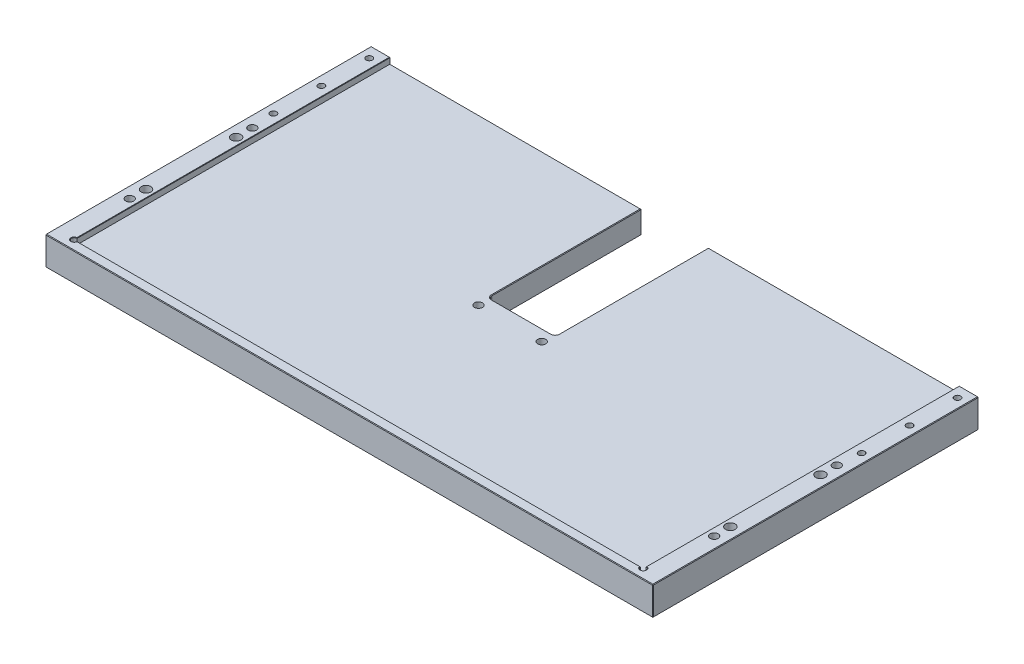
SolidWorks part; units mm, degrees
material "Al6061"
ref_plane "Front" through (0, 0, 0) normal (0, 0, 1) x (1, 0, 0)
ref_plane "Top" through (0, 0, 0) normal (0, 1, 0) x (1, 0, 0)
ref_plane "Right" through (0, 0, 0) normal (1, 0, 0) x (0, 0, -1)
sketch "草图1" plane through (0, 0, 0) normal (0, 1, 0) x (1, 0, 0)
  line L1 (-158.5, 85) -> (158.5, 85)
  line L2 (-158.5, 85) -> (-158.5, -85)
  line L3 (-158.5, -85) -> (158.5, -85)
  line L4 (158.5, 85) -> (158.5, -85)
  line L5 (-158.5, 85) -> (158.5, -85) construction
  line L6 (-158.5, -85) -> (158.5, 85) construction
  point P0 (0, 0)
  dimension "D1" = 317
  dimension "D2" = 170
extrude "凸台-拉伸1" add sketch "草图1" along normal blind 15
sketch "草图2" plane through (0, 15, 0) normal (0, 1, 0) x (1, 0, 0)
  line L0 (158.5, 85) -> (-158.5, 85) construction
  line L1 (-148.5, 250) -> (148.5, 250)
  line L2 (-148.5, 250) -> (-148.5, -80)
  line L3 (-148.5, -80) -> (148.5, -80)
  line L4 (148.5, 250) -> (148.5, -80)
  line L5 (-148.5, 250) -> (148.5, -80) construction
  line L6 (-148.5, -80) -> (148.5, 250) construction
  line L7 (158.5, -85) -> (158.5, 85) construction
  line L8 (-158.5, -85) -> (158.5, -85) construction
  point P0 (0, 85)
  dimension "D1" = 10
  dimension "D2" = 5
extrude "切除-拉伸1" cut sketch "草图2" against normal blind 3.1
sketch "草图3" plane through (0, 0, 0) normal (0, -1, 0) x (1, 0, 0)
  line L0 (0, 0) -> (0, -56.7771) construction
  line L1 (-17.5, -5) -> (17.5, -5)
  line L2 (-17.5, -5) -> (-17.5, -108.5542)
  line L3 (-17.5, -108.5542) -> (17.5, -108.5542)
  line L4 (17.5, -5) -> (17.5, -108.5542)
  line L5 (-17.5, -5) -> (17.5, -108.5542) construction
  line L6 (-17.5, -108.5542) -> (17.5, -5) construction
  line L7 (158.5, -85) -> (-158.5, -85) construction
  point P0 (0, -56.7771)
  dimension "D1" = 80
  dimension "D2" = 35
extrude "切除-拉伸2" cut sketch "草图3" against normal through all
hole_wizard "M5 螺纹孔1" positions "草图5" profile "草图4" tap size "M5" standard "Iso"
sketch "草图5" plane through (0, 0, 0) normal (0, -1, 0) x (-1, 0, 0)
  line L0 (0, 0) -> (0, -26.6863) construction
  line L2 (-17.5, 5) -> (17.5, 5) construction
  point P0 (-16.5, -1)
  point P2 (16.5, -1)
  dimension "D1" = 33
  dimension "D2" = 6
sketch "草图4" plane through (16.5, 0, 1) normal (1, 0, 0) x (0, 0, -1)
  line L0 (0, 0) -> (0, 17.2618)
  line L1 (0, 17.2618) -> (2.1, 16)
  line L2 (2.1, 16) -> (2.1, 0)
  line L5 (2.1, 0) -> (0, 0)
  line L10 (0, 17.2618) -> (-2.1, 16) construction
  line L11 (0, -6.35) -> (0, 107.95) construction
  dimension "螺纹孔钻头直径" = 4.2
  dimension "螺纹孔钻头深度" = 16
  dimension "导头角度" = 118
cosmetic thread "孔螺蚊线1" parameters "D1"=11.9, "D2"=5
cosmetic thread "孔螺蚊线2" parameters "D1"=11.9, "D2"=5
fillet "圆角1" radius 2 2 edges at (17.5, 5.95, -5) (-17.5, 5.95, -5)
sketch "草图6" plane through (0, 15, 0) normal (0, 1, 0) x (1, 0, 0)
  circle A0 centre (-148.5, -80) radius 1.5
  circle A1 centre (148.5, -80) radius 1.5
  dimension "D1" = 3
extrude "切除-拉伸3" cut sketch "草图6" against normal blind 5
chamfer "倒角1" distance 0.3 angle 45 30 edges at (17.5, 0, -46) (17.5, 11.9, -46) (16.9142, 0, -5.5858) (16.9142, 11.9, -5.5858) (0, 0, -5) (0, 11.9, -5) (-16.9142, 0, -5.5858) (-16.9142, 11.9, -5.5858) (-158.5, 15, 0) (-158.5, 7.5, 85) (0, 15, 85) (158.5, 7.5, 85) (158.5, 15, 0) (158.5, 7.5, -85) (153.5, 15, -85) (148.5, 13.45, -85) (83, 11.9, -85) (17.5, 5.95, -85) (88, 0, -85) (158.5, 0, 0) (0, 0, 85) (-158.5, 0, 0) (-148.5, 13.45, -85) (-153.5, 15, -85) (-158.5, 7.5, -85) (-88, 0, -85) (-83, 11.9, -85) (-17.5, 0, -46) (-17.5, 5.95, -85) (-17.5, 11.9, -46)
hole_wizard "M5 螺纹孔2" positions "草图8" profile "草图7" tap size "M5" standard "Iso" end condition through all
sketch "草图8" plane through (0, 15, 0) normal (0, 1, 0) x (1, 0, 0)
  line L0 (-158.5, -84.7) -> (-158.5, 84.7) construction
  line L2 (158.5, 84.7) -> (158.5, -84.7) construction
  line L3 (158.2, -85) -> (-158.2, -85) construction
  point P0 (152.5, 17)
  point P2 (152.5, -47)
  point P4 (-152.5, 17)
  point P6 (-152.5, -47)
  dimension "D1" = 6
  dimension "D2" = 64
  dimension "D3" = 38
  dimension "D4" = 6
cosmetic thread "孔螺蚊线3" parameters "D2"=5
cosmetic thread "孔螺蚊线4" parameters "D2"=5
cosmetic thread "孔螺蚊线5" parameters "D2"=5
cosmetic thread "孔螺蚊线6" parameters "D2"=5
sketch "草图7" plane through (152.5, 15, -17) normal (1, 0, 0) x (0, 0, 1)
  line L0 (0, 0) -> (0, 15)
  line L1 (0, 15) -> (2.1, 15)
  line L2 (2.1, 15) -> (2.1, 0)
  line L5 (2.1, 0) -> (0, 0)
  line L11 (0, -6.35) -> (0, 107.95) construction
  dimension "通孔螺纹孔钻头直径" = 4.2
  dimension "通孔螺纹孔钻头深度" = 15
hole_wizard "M4 螺纹孔1" positions "草图10" profile "草图9" tap size "M4" standard "Iso"
sketch "草图10" plane through (0, 15, 0) normal (0, 1, 0) x (1, 0, 0)
  line L0 (158.5, 84.7) -> (158.5, -84.7) construction
  line L1 (148.8, 85) -> (158.2, 85) construction
  line L2 (-158.5, -84.7) -> (-158.5, 84.7) construction
  point P0 (153.5, 79)
  point P2 (153.5, 54)
  point P4 (153.5, 29)
  point P10 (-153.5, 29)
  point P12 (-153.5, 54)
  point P14 (-153.5, 79)
  dimension "D1" = 5
  dimension "D2" = 6
  dimension "D3" = 25
  dimension "D4" = 25
  dimension "D5" = 5
sketch "草图9" plane through (153.5, 15, -79) normal (1, 0, 0) x (0, 0, 1)
  line L0 (0, 0) -> (0, 14.4914)
  line L1 (0, 14.4914) -> (1.65, 13.5)
  line L2 (1.65, 13.5) -> (1.65, 0)
  line L5 (1.65, 0) -> (0, 0)
  line L10 (0, 14.4914) -> (-1.65, 13.5) construction
  line L11 (0, -6.35) -> (0, 107.95) construction
  dimension "螺纹孔钻头直径" = 3.3
  dimension "螺纹孔钻头深度" = 13.5
  dimension "导头角度" = 118
cosmetic thread "孔螺蚊线7" parameters "D1"=10, "D2"=4
cosmetic thread "孔螺蚊线8" parameters "D1"=10, "D2"=4
cosmetic thread "孔螺蚊线9" parameters "D1"=10, "D2"=4
cosmetic thread "孔螺蚊线10" parameters "D1"=10, "D2"=4
cosmetic thread "孔螺蚊线11" parameters "D1"=10, "D2"=4
cosmetic thread "孔螺蚊线12" parameters "D1"=10, "D2"=4
sketch "草图11" plane through (0, 15, 0) normal (0, 1, 0) x (1, 0, 0)
  line L0 (-152.5, 17) -> (-152.5, -47) construction
  line L1 (152.5, 17) -> (152.5, -47) construction
  circle A0 centre (152.5, 8.5) radius 2.5
  circle A1 centre (152.5, -38.5) radius 2.5
  circle A2 centre (-152.5, 8.5) radius 2.5
  circle A3 centre (-152.5, -38.5) radius 2.5
  circle A4 centre (152.5, 17) radius 2.1 construction
  circle A5 centre (152.5, -47) radius 2.1 construction
  dimension "D1" = 8.5
  dimension "D2" = 8.5
  dimension "D3" = 5
extrude "切除-拉伸4" cut sketch "草图11" against normal blind 10
sketch "草图12" plane through (0, 15, 0) normal (0, 1, 0) x (1, 0, 0)
  circle A0 centre (152.5, 8.5) radius 1.5
  circle A1 centre (152.5, -38.5) radius 1.5
  circle A2 centre (-152.5, 8.5) radius 1.5
  circle A3 centre (-152.5, -38.5) radius 1.5
  dimension "D1" = 3
extrude "切除-拉伸5" cut sketch "草图12" against normal through all
hole_wizard "M4 螺纹孔2" positions "草图14" profile "草图13" tap size "M4" standard "Iso"
sketch "草图14" plane through (0, 0, 0) normal (0, -1, 0) x (-1, 0, 0)
  line L0 (158.2, -85) -> (-158.2, -85) construction
  line L1 (158.5, 84.7) -> (158.5, -84.7) construction
  line L2 (-158.5, -84.7) -> (-158.5, 84.7) construction
  point P0 (148.5, 25)
  point P2 (148.5, -55)
  point P4 (108.5, 25)
  point P6 (108.5, -55)
  point P8 (-148.5, 25)
  point P10 (-108.5, 25)
  point P12 (-148.5, -55)
  point P14 (-108.5, -55)
  dimension "D1" = 30
  dimension "D2" = 40
  dimension "D3" = 80
  dimension "D4" = 10
  dimension "D5" = 10
  dimension "D6" = 40
cosmetic thread "孔螺蚊线13" parameters "D1"=7, "D2"=4
cosmetic thread "孔螺蚊线14" parameters "D1"=7, "D2"=4
cosmetic thread "孔螺蚊线15" parameters "D1"=7, "D2"=4
cosmetic thread "孔螺蚊线16" parameters "D1"=7, "D2"=4
cosmetic thread "孔螺蚊线17" parameters "D1"=7, "D2"=4
cosmetic thread "孔螺蚊线18" parameters "D1"=7, "D2"=4
cosmetic thread "孔螺蚊线19" parameters "D1"=7, "D2"=4
cosmetic thread "孔螺蚊线20" parameters "D1"=7, "D2"=4
sketch "草图13" plane through (-148.5, 0, -25) normal (1, 0, 0) x (0, 0, -1)
  line L0 (0, 0) -> (0, 9.9914)
  line L1 (0, 9.9914) -> (1.65, 9)
  line L2 (1.65, 9) -> (1.65, 0)
  line L5 (1.65, 0) -> (0, 0)
  line L10 (0, 9.9914) -> (-1.65, 9) construction
  line L11 (0, -6.35) -> (0, 107.95) construction
  dimension "螺纹孔钻头直径" = 3.3
  dimension "螺纹孔钻头深度" = 9
  dimension "导头角度" = 118
chamfer "倒角3" distance 0.2 angle 45 5 edges at (-148.5, 15, -3.1) (-149.5607, 15, 81.0607) (0, 15, 80) (149.5607, 15, 81.0607) (148.5, 15, -3.1)
